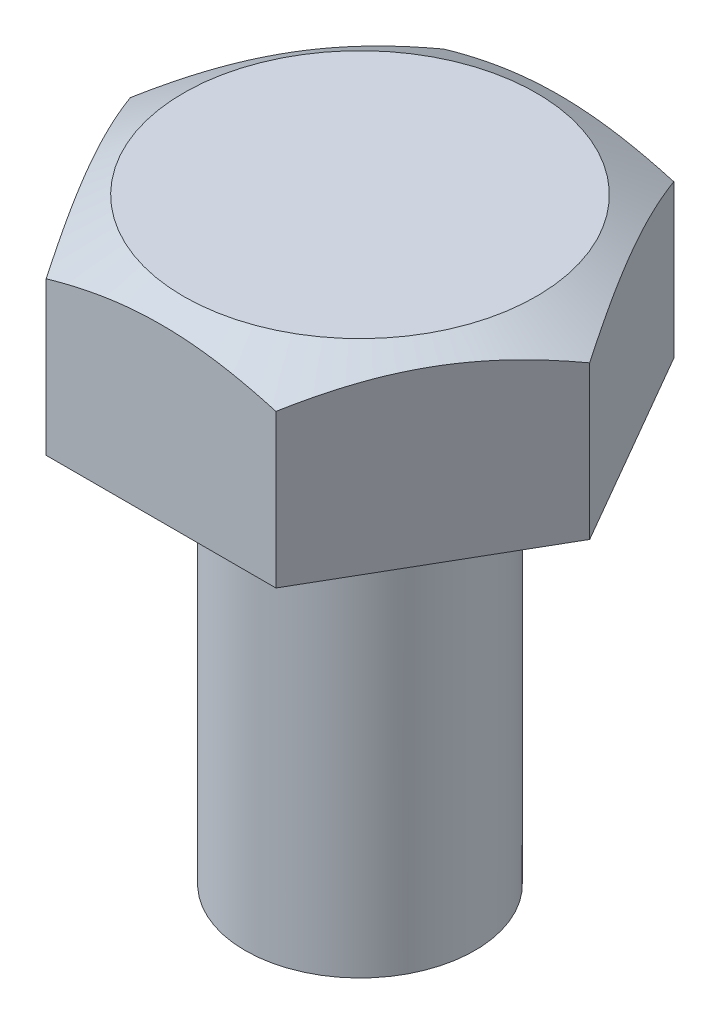
from build123d import *

# Parameters (mm, degrees)
BOSS_EXTRUDE1_DEPTH = 4
SKETCH2_OUTSIDE_W   = 45.006
SKETCH2_OUTSIDE_H   = 43.666
SKETCH2_OUTSIDE_R   = 3.838579207
CUT_EXTRUDE1_DEPTH  = 8.729812417
CUT_EXTRUDE1_DRAFT  = -60
SKETCH3_R           = 2.5
BOSS_EXTRUDE2_DEPTH = 9


with BuildPart() as part:
    # Sketch1 → Boss-Extrude1 (new body)
    with BuildSketch(Plane(origin=(0, 0, 0), x_dir=(1, 0, 0), z_dir=(0, 1, 0))):
        Polygon((5, 0), (2.5, 4.330127019), (-2.5, 4.330127019), (-5, 0), (-2.5, -4.330127019), (2.5, -4.330127019), align=None)
    extrude(amount=BOSS_EXTRUDE1_DEPTH)


with BuildPart() as cut_extrude1_tool:
    # Sketch2 outside → Cut-Extrude1 (with draft: the straight prism first)
    with BuildSketch(Plane(origin=(0, 4, 0), x_dir=(1, 0, 0), z_dir=(0, 1, 0))):
        Rectangle(SKETCH2_OUTSIDE_W, SKETCH2_OUTSIDE_H)
        Circle(SKETCH2_OUTSIDE_R, mode=Mode.SUBTRACT)
    extrude(amount=-CUT_EXTRUDE1_DEPTH)
    # Cut-Extrude1: the draft: its side faces are tilted about the plane it starts from
    cut_extrude1_sides = [cut_extrude1_tool.faces().sort_by_distance(p)[0] for p in [
        (0, -0.364906208, 21.833),
        (22.503, -0.364906208, 0),
        (0, -0.364906208, -21.833),
        (-22.503, -0.364906208, 0),
        (-3.838579207, -0.364906208, 0),
    ]]
    draft(cut_extrude1_sides, Plane(origin=(0, 4, 0), x_dir=(1, 0, 0), z_dir=(0, 1, 0)), CUT_EXTRUDE1_DRAFT)


with BuildPart() as part_1:
    add(part.part)

    # Cut-Extrude1: cut by cut_extrude1_tool
    add(cut_extrude1_tool.part, mode=Mode.SUBTRACT)

    # Sketch3 → Boss-Extrude2 (add)
    with BuildSketch(Plane.XZ):
        with Locations(Location((0, 0, 0), (0, 0, 90))):
            Circle(SKETCH3_R)
    extrude(amount=BOSS_EXTRUDE2_DEPTH)


solid = part_1.part
